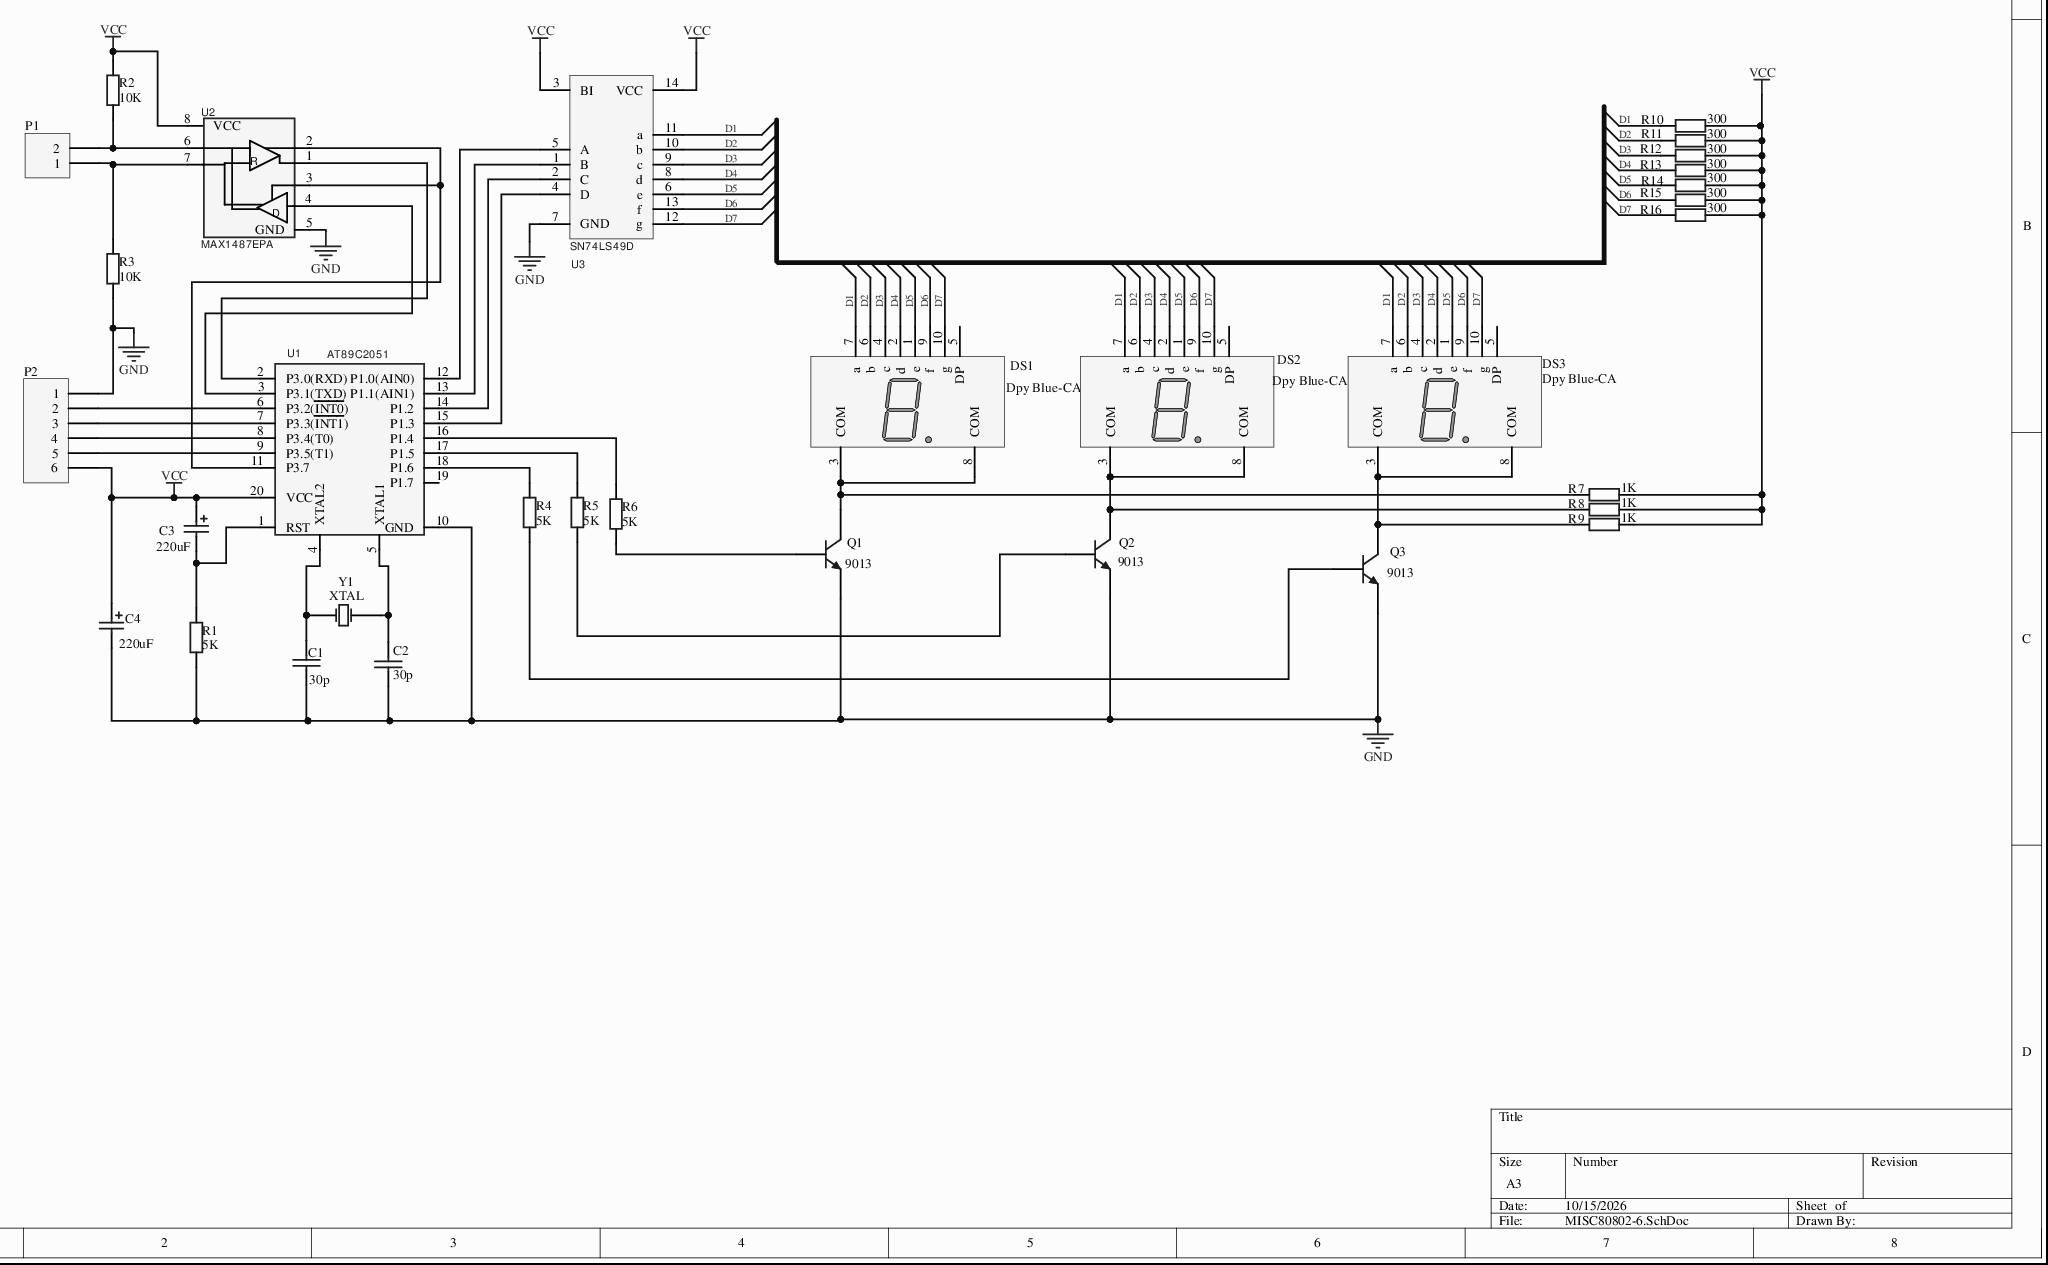
[diagram p0: MISC80802-6.SchDoc]
# Altium project MISC80802-7.PrjPcb
1 sheet, 32 parts. Net scope: global (net labels, ports and power ports of the same name join across sheets).
Board file: MISC80802.PcbDoc

## Sheet MISC80802-6.SchDoc
size A3

### Parts
C1  30p  [RAD-0.1]
C2  30p  [RAD-0.1]
C3  value 220uF  [CAPR5-4X5]  (hidden comment: Cap Pol2)
C4  value 220uF  [RB5-10.5]  (hidden comment: Cap Pol2)
DS1  Dpy Blue-CA  [H]
DS2  Dpy Blue-CA  [H]
DS3  Dpy Blue-CA  [H]
P1  Header 2  [HDR1X2]  (value not drawn)
P2  Header 6  [HDR1X6]  (value not drawn)
Q1  9013  [TO-92A]
Q2  9013  [TO-92A]
Q3  9013  [TO-92A]
R1  1: 5K  [AXIAL-0.4]  (hidden comment: Res2)
R2  1: 10K  [AXIAL-0.4]  (hidden comment: Res2)
R3  1: 10K  [AXIAL-0.4]  (hidden comment: Res2)
R4  1: 5K  [AXIAL-0.4]  (hidden comment: Res2)
R5  1: 5K  [AXIAL-0.4]  (hidden comment: Res2)
R6  1: 5K  [AXIAL-0.4]  (hidden comment: Res2)
R7  1: 1K  [AXIAL-0.4]  (hidden comment: Res2)
R8  1: 1K  [AXIAL-0.4]  (hidden comment: Res2)
R9  1: 1K  [AXIAL-0.4]  (hidden comment: Res2)
R10  1: 300  [AXIAL-0.4]  (hidden comment: Res2)
R11  1: 300  [AXIAL-0.4]  (hidden comment: Res2)
R12  1: 300  [AXIAL-0.4]  (hidden comment: Res2)
R13  1: 300  [AXIAL-0.4]  (hidden comment: Res2)
R14  1: 300  [AXIAL-0.4]  (hidden comment: Res2)
R15  1: 300  [AXIAL-0.4]  (hidden comment: Res2)
R16  1: 300  [AXIAL-0.4]  (hidden comment: Res2)
U1  AT89C2051  [DIP20]
U2  MAX1487EPA  [PA8]
U3  SN74LS49D  [SOP14]
Y1  XTAL  [R38]

### Nets
GND: C1.2 C2.2 C4.2 P2.1 Q1.1(E) Q2.1(E) Q3.1(E) R1.1 R3.1 U1.10(GND) U2.5(GND) U3.7(GND)
VCC: C3.1 C4.1 P2.6 R2.2 R7.1 R8.1 R9.1 R10.1 R11.1 R12.1 R13.1 R14.1 R15.1 R16.1 U1.20(VCC) U2.8(VCC) U3.3(BI) U3.14(VCC)
D1: DS1.7(a) DS2.7(a) DS3.7(a) R10.2 U3.11(a)
D2: DS1.6(b) DS2.6(b) DS3.6(b) R11.2 U3.10(b)
D3: DS1.4(c) DS2.4(c) DS3.4(c) R12.2 U3.9(c)
D4: DS1.2(d) DS2.2(d) DS3.2(d) R13.2 U3.8(d)
D5: DS1.1(e) DS2.1(e) DS3.1(e) R14.2 U3.6(e)
D6: DS1.9(f) DS2.9(f) DS3.9(f) R15.2 U3.13(f)
D7: DS1.10(g) DS2.10(g) DS3.10(g) R16.2 U3.12(g)
NetC1_1: C1.1 U1.4(XTAL2) Y1.1(OSC1)
NetC2_1: C2.1 U1.5(XTAL1) Y1.2(OSC2)
NetC3_2: C3.2 R1.2 U1.1(RST)
NetDS1_3: DS1.3(COM) DS1.8(COM) Q1.3(C) R7.2
NetDS2_3: DS2.3(COM) DS2.8(COM) Q2.3(C) R8.2
NetDS3_3: DS3.3(COM) DS3.8(COM) Q3.3(C) R9.2
NetP1_1: P1.1 R3.2 U2.7(B)
NetP1_2: P1.2 R2.1 U2.6(A)
NetP2_2: P2.2 U1.6(P3.2(~{INT0}))
NetP2_3: P2.3 U1.7(P3.3(~{INT1}))
NetP2_4: P2.4 U1.8(P3.4(T0))
NetP2_5: P2.5 U1.9(P3.5(T1))
NetQ1_2: Q1.2(B) R6.1
NetQ2_2: Q2.2(B) R5.1
NetQ3_2: Q3.2(B) R4.1
NetR4_2: R4.2 U1.18(P1.6)
NetR5_2: R5.2 U1.17(P1.5)
NetR6_2: R6.2 U1.16(P1.4)
NetU1_2: U1.2(P3.0(RXD)) U2.1(RO)
NetU1_3: U1.3(P3.1(TXD)) U2.4(DI)
NetU1_11: U1.11(P3.7) U2.2(RE#) U2.3(DE)
NetU1_12: U1.12(P1.0(AIN0)) U3.5(A)
NetU1_13: U1.13(P1.1(AIN1)) U3.1(B)
NetU1_14: U1.14(P1.2) U3.2(C)
NetU1_15: U1.15(P1.3) U3.4(D)

Not connected (* = marked no-connect by the designer): DS1 5(DP); DS2 5(DP); DS3 5(DP); U1 19(P1.7)

### Library data of the parts
C1 C2 = 瓷片电容
C3 C4 = Cap Pol2: Polarized Capacitor (Axial); Published: 8-Jun-2000; LatestRevisionDate: 17-Jul-2002; LatestRevisionNote: Re-released for DXP Platform.; PackageReference: POLAR0.8; PackageDescription: Polarized Capacitor; 2 Leads; Publisher: Altium Limited
DS1-DS3 = Dpy Blue-CA: 14.2 mm General Purpose Blue 7-Segment Display: CA, RH DP, Gray Surface; MinimumIntensity: 2020 ucd; Note: IF = 10 mA; Published: 8-Jun-2000; LatestRevisionDate: 17-Dec-2003; LatestRevisionNote: Schematic revised, PCB Footprint replaced.; DatasheetVersion: 24-Sep-2002; PackageVersion: 24-Sep-2002; PackageReference: H; PackageDescription: LED, 7-Segment Display, 14.2 mm, RHD; 10 Leads; Row Space 15.24 mm; Pitch 2.54 mm; Colour: Blue; ComponentLink1Description: Manufacturer Link; Publisher: Altium Limited
P1 = Header 2: Header, 2-Pin; LatestRevisionDate: 17-Jul-2002; LatestRevisionNote: Re-released for DXP Platform.; Publisher: Altium Limited
P2 = Header 6: Header, 6-Pin; LatestRevisionDate: 17-Jul-2002; LatestRevisionNote: Re-released for DXP Platform.; Publisher: Altium Limited
Q1-Q3 = 2N3904: NPN General Purpose Amplifier; Published: 8-Jun-2000; LatestRevisionDate: 15-Jan-2003; LatestRevisionNote: PCB Footprint 'BCY-W3/D4.7' replaced; DatasheetVersion: 1997; PackageVersion: Sep-1998; PackageReference: TO-92A; PackageDescription: TO, Flat Index; 3 In-Line, Axial Leads; Body Dia. 4.5mm; Leads 0.51 x 0.48 mm (max); ComponentLink1Description: Manufacturer Link; ComponentLink2Description: Datasheet; ComponentLink2URL: http://www.fairchildsemi.com/ds/2N%2F2N3904.pdf; Publisher: Altium Limited
R1-R16 = Res2: Resistor; Published: 8-Jun-2000; LatestRevisionDate: 17-Jul-2002; LatestRevisionNote: Re-released for DXP Platform.; PackageReference: AXIAL-0.4; PackageDescription: Axial Device, Thru-Hole; 2 Leads; 0.4 in Pin Spacing; Publisher: Altium Limited
U1 = AT89C2051-24PU
Y1 = XTAL: Crystal Oscillator; Published: 8-Jun-2000; LatestRevisionDate: 17-Jul-2002; LatestRevisionNote: Re-released for DXP Platform.; PackageReference: R38; PackageDescription: Crystal, Thru-Hole; 2 Leads; Body 3.1 x 8.2 mm (Dia.xH); Publisher: Altium Limited